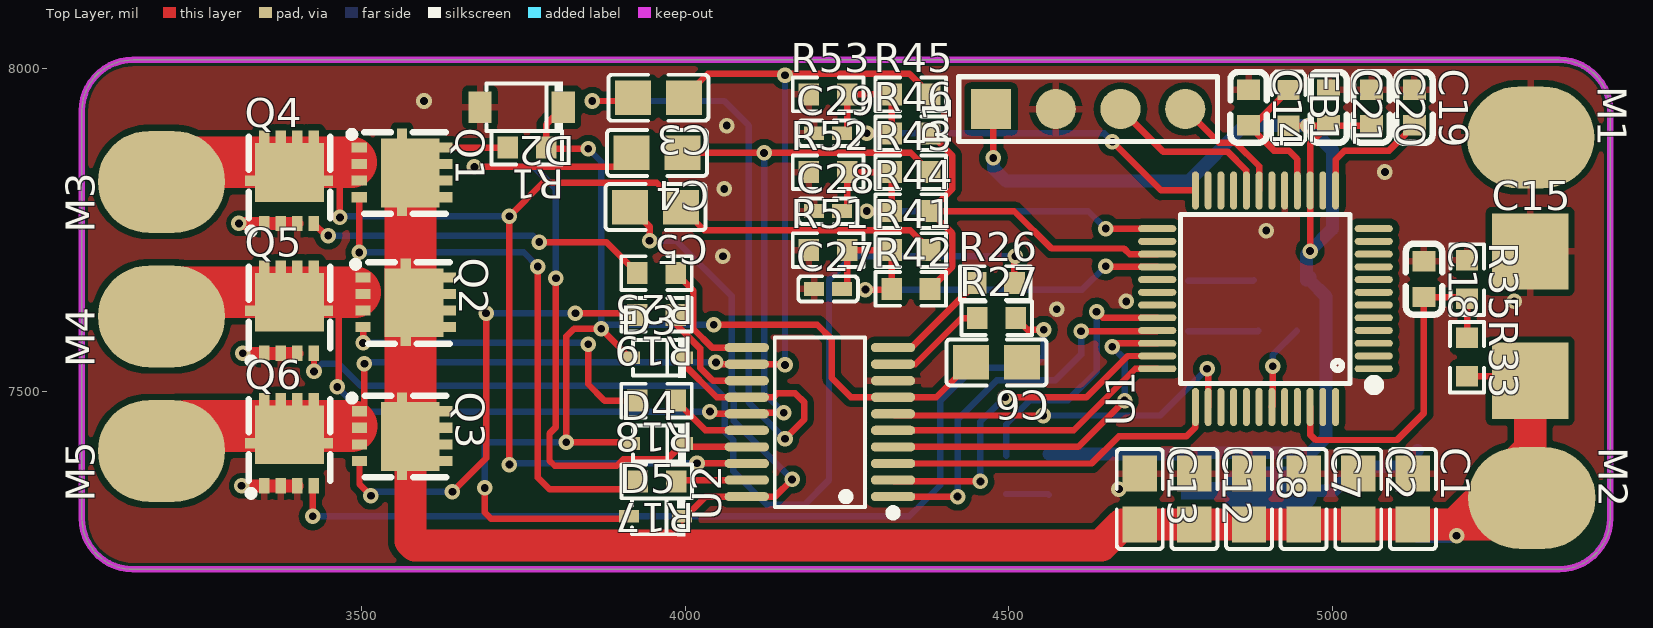
[diagram p0: Top Layer view]
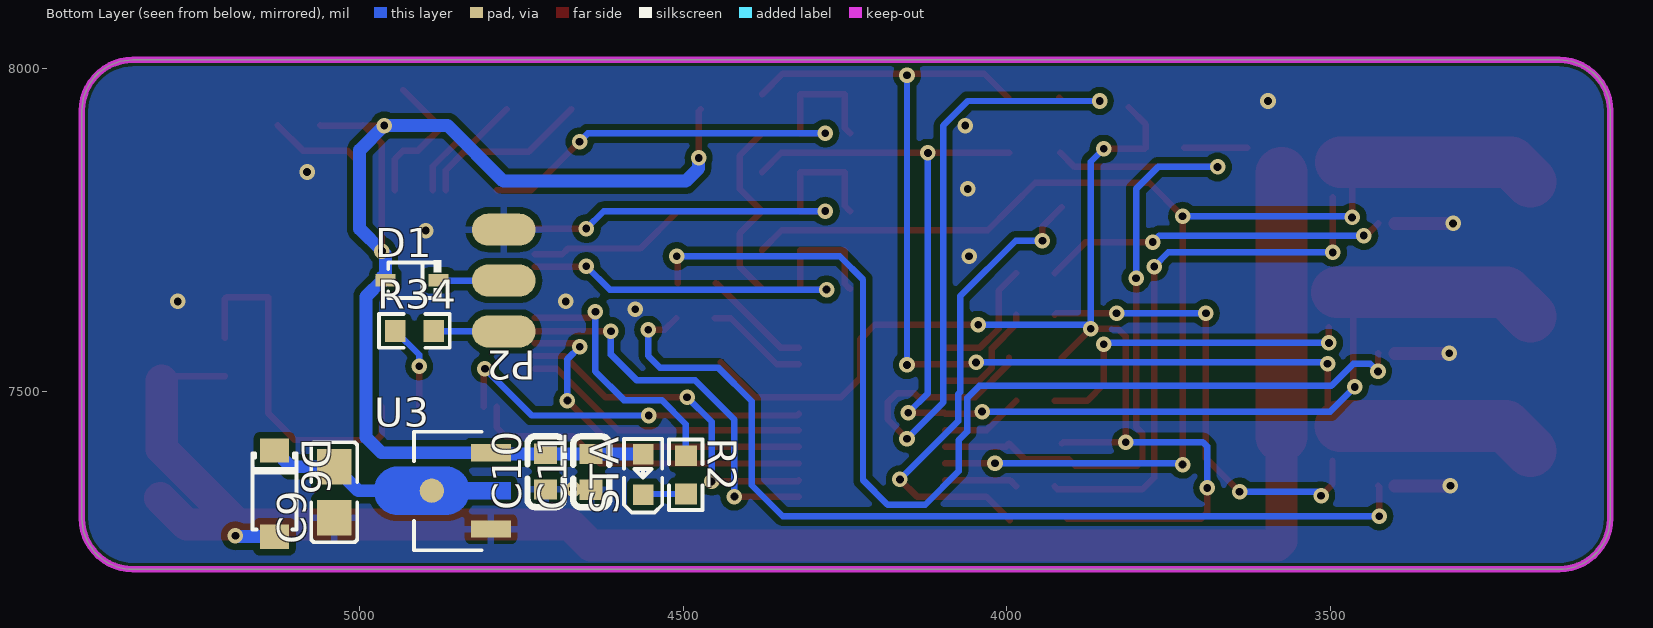
[diagram p1: Bottom Layer view, seen from below]
# Altium PCB MISC52085.pcbdoc
Units mil, origin at the board's own origin, x right, y up, seen from the top; angles counter-clockwise.
Board outline 2362.2 x 787.4 mil, 2 copper layers (Top Layer, Bottom Layer), stack 62.206 mil thick; 66 components, 45 nets, 249 pads, 70 vias.

## Layer stack, top to bottom
Top Solder Mask Layer: solder mask 0.394, Dk 3.3
Top Layer: signal copper 1.379
Dielectric1: surface 59.449, FR4, Dk 4.5
Bottom Layer: signal copper 1.378
Bottom Solder Mask Layer: solder mask 0.394, Dk 3.3

## Board outline
3067.18,7304.15 ccw(c3145.92,7304.15) 3145.92,7225.41 5350.64,7225.41 ccw(c5350.64,7304.15) 5429.38,7304.15 5429.38,7934.07 ccw(c5350.64,7934.07) 5350.64,8012.81 3145.92,8012.81 ccw(c3145.92,7934.07) 3067.18,7934.07

## Design rules (kind name [scope] priority, off if disabled: settings)
BoardOutlineClearance copperThickness2oz_1 [All] p2 off: genericclearance=7.99 ignorepadtopadclearanceinfootprint=FALSE except(0: Arc-SplitContinuation Track-SplitContinuation SMDPad-SplitContinuation THPad-SplitContinuation Via-SplitContinuation Fill-SplitContinuation Region-SplitContinuation Poly-SplitContinuation Text-SplitContinuation Hole-SplitContinuation; 5.98: Arc-CutoutEdge Track-CutoutEdge SMDPad-CutoutEdge THPad-CutoutEdge Via-CutoutEdge Text-CutoutEdge; 6.89: Hole-OutlineEdge Hole-CutoutEdge; 10: Poly-OutlineEdge Poly-CutoutEdge; 11.81: Arc-OutlineEdge Track-OutlineEdge SMDPad-OutlineEdge THPad-OutlineEdge Via-OutlineEdge Fill-OutlineEdge Region-OutlineEdge Text-OutlineEdge Fill-CutoutEdge Region-CutoutEdge)
BoardOutlineClearance Plane_innerPlane_1 [All] p4 off: genericclearance=4.02 ignorepadtopadclearanceinfootprint=FALSE except(0: Arc-SplitContinuation Track-SplitContinuation SMDPad-SplitContinuation THPad-SplitContinuation Via-SplitContinuation Fill-SplitContinuation Region-SplitContinuation Poly-SplitContinuation Text-SplitContinuation Hole-SplitContinuation; 5.98: Arc-CutoutEdge Track-CutoutEdge SMDPad-CutoutEdge THPad-CutoutEdge Via-CutoutEdge Text-CutoutEdge; 6.89: Hole-OutlineEdge Hole-CutoutEdge; 10: Poly-OutlineEdge Poly-CutoutEdge; 11.81: Arc-OutlineEdge Track-OutlineEdge SMDPad-OutlineEdge THPad-OutlineEdge Via-OutlineEdge Fill-OutlineEdge Region-OutlineEdge Text-OutlineEdge Fill-CutoutEdge Region-CutoutEdge)
BoardOutlineClearance Copper_copperRegion_1 [All] p6 off: genericclearance=4.02 ignorepadtopadclearanceinfootprint=FALSE except(0: Arc-SplitContinuation Track-SplitContinuation SMDPad-SplitContinuation THPad-SplitContinuation Via-SplitContinuation Fill-SplitContinuation Region-SplitContinuation Poly-SplitContinuation Text-SplitContinuation Hole-SplitContinuation; 5.98: Arc-CutoutEdge Track-CutoutEdge SMDPad-CutoutEdge THPad-CutoutEdge Via-CutoutEdge Text-CutoutEdge; 6.89: Hole-OutlineEdge Hole-CutoutEdge; 10: Poly-OutlineEdge Poly-CutoutEdge; 11.81: Arc-OutlineEdge Track-OutlineEdge SMDPad-OutlineEdge THPad-OutlineEdge Via-OutlineEdge Fill-OutlineEdge Region-OutlineEdge Text-OutlineEdge Fill-CutoutEdge Region-CutoutEdge)
BoardOutlineClearance copperThickness1oz_1 [All] p8: genericclearance=4.02 ignorepadtopadclearanceinfootprint=FALSE except(0: Arc-SplitContinuation Track-SplitContinuation SMDPad-SplitContinuation THPad-SplitContinuation Via-SplitContinuation Fill-SplitContinuation Region-SplitContinuation Poly-SplitContinuation Text-SplitContinuation Hole-SplitContinuation; 5.98: Arc-CutoutEdge Track-CutoutEdge SMDPad-CutoutEdge THPad-CutoutEdge Via-CutoutEdge Text-CutoutEdge; 6.89: Hole-OutlineEdge Hole-CutoutEdge; 10: Poly-OutlineEdge Poly-CutoutEdge; 11.81: Arc-OutlineEdge Track-OutlineEdge SMDPad-OutlineEdge THPad-OutlineEdge Via-OutlineEdge Fill-OutlineEdge Region-OutlineEdge Text-OutlineEdge Fill-CutoutEdge Region-CutoutEdge)
Clearance copperThickness2oz [All] p1 off: gap=7.99 ignorepadtopadclearanceinfootprint=FALSE except(5.98: SMDPad-Track SMDPad-SMDPad THPad-Track SMDPad-THPad THPad-THPad Track-Via SMDPad-Via THPad-Via Via-Via Fill-SMDPad Region-SMDPad Fill-THPad Region-THPad Fill-Via Region-Via Fill-Fill Fill-Region Region-Region Arc-Track Arc-SMDPad Arc-THPad Arc-Via Fill-Arc Region-Arc Arc-Arc Text-Track SMDPad-Text Text-THPad Text-Via Fill-Text Region-Text Arc-Text Text-Text; 6.89: Hole-Track Hole-SMDPad Hole-THPad Hole-Via Fill-Hole Region-Hole Hole-Arc Hole-Text; 10: Poly-Track Poly-SMDPad Poly-THPad Poly-Via Poly-Fill Poly-Region Poly-Poly Poly-Arc Poly-Text Poly-Hole; 11.81: Fill-Track Region-Track)
Clearance Plane_innerPlane [All] p3 off: gap=4.02 ignorepadtopadclearanceinfootprint=FALSE except(5.98: SMDPad-Track SMDPad-SMDPad THPad-Track SMDPad-THPad THPad-THPad Track-Via SMDPad-Via THPad-Via Via-Via Fill-SMDPad Region-SMDPad Fill-THPad Region-THPad Fill-Via Region-Via Fill-Fill Fill-Region Region-Region Arc-Track Arc-SMDPad Arc-THPad Arc-Via Fill-Arc Region-Arc Arc-Arc Text-Track SMDPad-Text Text-THPad Text-Via Fill-Text Region-Text Arc-Text Text-Text; 6.89: Hole-Track Hole-SMDPad Hole-THPad Hole-Via Fill-Hole Region-Hole Hole-Arc Hole-Text; 10: Poly-Track Poly-SMDPad Poly-THPad Poly-Via Poly-Fill Poly-Region Poly-Poly Poly-Arc Poly-Text Poly-Hole; 11.81: Fill-Track Region-Track)
Clearance Copper_copperRegion [All] p5 off: gap=4.02 ignorepadtopadclearanceinfootprint=FALSE except(5.98: SMDPad-Track SMDPad-SMDPad THPad-Track SMDPad-THPad THPad-THPad Track-Via SMDPad-Via THPad-Via Via-Via Fill-SMDPad Region-SMDPad Fill-THPad Region-THPad Fill-Via Region-Via Fill-Fill Fill-Region Region-Region Arc-Track Arc-SMDPad Arc-THPad Arc-Via Fill-Arc Region-Arc Arc-Arc Text-Track SMDPad-Text Text-THPad Text-Via Fill-Text Region-Text Arc-Text Text-Text; 6.89: Hole-Track Hole-SMDPad Hole-THPad Hole-Via Fill-Hole Region-Hole Hole-Arc Hole-Text; 10: Poly-Track Poly-SMDPad Poly-THPad Poly-Via Poly-Fill Poly-Region Poly-Poly Poly-Arc Poly-Text Poly-Hole; 11.81: Fill-Track Region-Track)
Clearance copperThickness1oz [All] p7: gap=4.02 ignorepadtopadclearanceinfootprint=FALSE except(5.98: SMDPad-Track SMDPad-SMDPad THPad-Track SMDPad-THPad THPad-THPad Track-Via SMDPad-Via THPad-Via Via-Via Fill-SMDPad Region-SMDPad Fill-THPad Region-THPad Fill-Via Region-Via Fill-Fill Fill-Region Region-Region Arc-Track Arc-SMDPad Arc-THPad Arc-Via Fill-Arc Region-Arc Arc-Arc Text-Track SMDPad-Text Text-THPad Text-Via Fill-Text Region-Text Arc-Text Text-Text; 6.89: Hole-Track Hole-SMDPad Hole-THPad Hole-Via Fill-Hole Region-Hole Hole-Arc Hole-Text; 10: Poly-Track Poly-SMDPad Poly-THPad Poly-Via Poly-Fill Poly-Region Poly-Poly Poly-Arc Poly-Text Poly-Hole; 11.81: Fill-Track Region-Track)
DiffPairsRouting differentialPair [All] p1: maxlimit=6 minlimit=6 mostfreqgap=6 toplayer_minwidth=5 toplayer_prefwidth=10 toplayer_maxwidth=100 toplayer_mingap=6 toplayer_prefgap=6 toplayer_maxgap=6 bottomlayer_minwidth=5 bottomlayer_prefwidth=10 bottomlayer_maxwidth=100 bottomlayer_mingap=6 bottomlayer_prefgap=6 bottomlayer_maxgap=6 maxuncoupledlength=10
HoleToHoleClearance otherClearance [All] p1: gap=11.81 allowstackedmicrovias=TRUE
Length netLength [All] p1: minlimit=0 maxlimit=0
PasteMaskExpansion pasteMaskExpansion [All] p1: expansion=0
PlaneConnect innerPlane [All] p1: planeconnectstyle=Relief reliefexpansion=20 reliefentries=4 reliefconductorwidth=10 reliefairgap=10
PolygonConnect copperRegion [All] p1: connectstyle=Relief reliefconductorwidth=10 reliefentries=4 polygonreliefangle="90 Angle" airgapwidth=10 via.connectstyle=Relief via.reliefconductorwidth=10 via.reliefentries=4 via.polygonreliefangle="90 Angle" via.airgapwidth=10
RoutingVias viaSize [All] p1: holewidth=12.01 width=24.02 viastyle="Through Hole" minholewidth=11.81 minwidth=19.68 maxholewidth=248.03 maxwidth=393.7
SolderMaskExpansion solderMaskExpansion [IsVia] p1: expansion=-1000 istentingtop=TRUE
SolderMaskExpansion solderMaskExpansion [All] p2: expansion=2.01 istentingtop=FALSE
Width copperThickness2oz_2 [All] p1 off: maxlimit=100 minlimit=8 preferedwidth=10
Width copperThickness1oz_2 [All] p2: maxlimit=100 minlimit=5 preferedwidth=10

## Components (designator, comment, footprint, x,y, rotation, side; value= is the part's Value field where it differs from the comment)
C1 "22uF" C0805 5124.51,7333.92 r270 top
C2 "22uF" C0805 5040.09,7333.92 r270 top
C3 "4.7uF" C0805 3958.24,7954.26 r180 top
C4 "4.7uF" C0805 3956.24,7869.04 r180 top
C5 "4.7uF" C0805 3954,7785.25 r180 top
C6 "22uF" C0805 4481.05,7545.28 r180 top
C7 "22uF" C0805 4955.66,7333.92 r270 top
C8 "22uF" C0805 4871.23,7333.92 r270 top
C9 "22uF" C0805 5039.24,7344.49 r90 bottom
C10 "10uF" C0603 4712.62,7376.35 r90 bottom
C11 "100nF" C0603 4642.14,7376.1 r90 bottom
C12 "22uF" C0805 4786.8,7333.92 r270 top
C13 "22uF" C0805 4702.37,7333.92 r270 top
C14 "100nF" C0603 4870.51,7939.35 r270 top
C15 "470uf" 焊盘 5305.72,7516.65 r0 top
C18 "100nF" C0603 5141.64,7673.78 r270 top
C19 "100nF" C0603 5126.94,7939.35 r270 top
C20 "10uF" C0603 5060.66,7939.35 r270 top
C21 "100nF" C0603 4994.38,7939.35 r270 top
C27 "100nF" C0402 4220.55,7658.77 r0 top
C28 "100nF" C0402 4220.55,7779.02 r0 top
C29 "100nF" C0402 4220.55,7899.28 r0 top
D1 "B5819WS" SOD-323_L1.7-W1.3-LS2.5-FD 4919.31,7672.15 r180 bottom
D2 "BZT52C15" SOD-123_L2.7-W1.6-LS3.7-RD 3747,7939.55 r180 top
D3 "B5819WS" SOD-323_L1.7-W1.3-LS2.5-FD 3955.39,7552.38 r0 top
D4 "B5819WS" SOD-323_L1.7-W1.3-LS2.5-FD 3955.39,7419.82 r0 top
D5 "B5819WS" SOD-323_L1.7-W1.3-LS2.5-FD 3954,7307.25 r0 top
D6 "DSK34" SOD-123_L2.8-W1.8-LS3.7-RD 5131.61,7342.48 r270 bottom
FB1 "MLB1608F-000T" L0603 4932.48,7938.69 r270 top
M1 "MountHole" 3*4焊盘 5306.45,7892.98 r270 top
M2 "MountHole" 3*4焊盘 5308.45,7335.61 r270 top
M3 "MountHole" 3*4焊盘 3190.27,7824.24 r90 top
M4 "MountHole" 3*4焊盘 3190.27,7616.24 r90 top
M5 "MountHole" 3*4焊盘 3190.27,7408.25 r90 top
P1 "Header-D-M 1x4P" 调试端口2.54_1X4 4617.58,7936.82 r90 top
P2 "Header-D-M 1x3P" 3P 4777.16,7671.73 r0 bottom
Q1 "TPN2R703NL,L1Q(M" TSON-8_L3.1-W3.1-P0.65-LS3.3-BL-EP 3561.99,7838.93 r270 top
Q2 "TPN2R703NL,L1Q(M" TSON-8_L3.1-W3.1-P0.65-LS3.3-BL-EP 3567.75,7638.14 r270 top
Q3 "TPN2R703NL,L1Q(M" TSON-8_L3.1-W3.1-P0.65-LS3.3-BL-EP 3562.24,7431.33 r270 top
Q4 "TPN2R703NL,L1Q(M" TSON-8_L3.1-W3.1-P0.65-LS3.3-BL-EP 3387.35,7825.95 r0 top
Q5 "TPN2R703NL,L1Q(M" TSON-8_L3.1-W3.1-P0.65-LS3.3-BL-EP 3387.35,7625.16 r0 top
Q6 "TPN2R703NL,L1Q(M" TSON-8_L3.1-W3.1-P0.65-LS3.3-BL-EP 3387.35,7420.36 r0 top
R1 "100Ω" R0603 3755.03,7877.3 r180 top
R2 "10kΩ" R0603 4495.84,7371.45 r270 bottom
R17 "4.7Ω" R0603 3956,7361.25 r180 top
R18 "4.7Ω" R0603 3955.39,7486.1 r180 top
R19 "4.7Ω" R0603 3955.39,7618.67 r180 top
R25 "4.7Ω" R0603 3955.39,7683.25 r180 top
R26 "4.7Ω" R0603 4479.04,7667.76 r0 top
R27 "4.7Ω" R0603 4481.05,7613.55 r0 top
R33 "47kΩ" R0603 5208.15,7553.3 r270 top
R34 "100Ω" R0603 4915.29,7593.84 r180 bottom
R35 "10kΩ" R0603 5208.36,7673.26 r270 top
R41 "5.1kΩ" R0603 4348.46,7718.9 r0 top
R42 "1kΩ" R0603 4348.46,7658.77 r0 top
R43 "5.1kΩ" R0603 4348.46,7839.15 r0 top
R44 "1kΩ" R0603 4348.46,7779.02 r0 top
R45 "5.1kΩ" R0603 4348.46,7959.41 r0 top
R46 "1kΩ" R0603 4348.46,7899.28 r0 top
R51 "1kΩ" R0603 4220.55,7718.9 r0 top
R52 "1kΩ" R0603 4220.55,7839.15 r0 top
R53 "1kΩ" R0603 4220.55,7959.41 r0 top
STA "LTST-C191KSKT" LED0603-RD-YELLOW 4561.65,7371.97 r90 bottom
U1 "STC32G8K64-42I-LQFP48" LQFP-48_L7.0-W7.0-P0.50-LS9.0-BL 4896.68,7643.66 r90 top
U2 "FD6288T" TSSOP-20_L6.5-W4.4-P0.65-LS6.4-BL 4207.97,7452.91 r90 top
U3 "SE8650KX-LF" SOT-89-3_L4.3-W2.3-P1.50-LS4.3-BR 4850.5,7346.5 r180 bottom

## Footprints (in the part's own frame and the unit in brackets; to place one, negate y for a bottom-side part, rotate by r counter-clockwise, add the part's x,y. Pads: shape width x height; smd on the part's side, far side on the other; paste and mask are expansions set on the pad)
3*4焊盘 [mm]
  oval 4x5 smd paste+0 mask+0.102: 1(0,0)
3P [mm]
  oval 2.5x1.25 smd paste+0 mask+0.051: 1(0,2) 2(0,0) 3(0,-2)
C0402 [mm]
  rect 0.79x0.54 smd paste-100 mask+0.051: 1(-0.545,0) 2(0.545,0)
  silkscreen extent -1.17,-0.5 1.17,0.5
C0603 [mm]
  rect 0.8x0.9 smd: 1(-0.7,0) 2(0.7,0)
  silkscreen extent -1.39,-0.71 1.39,0.71
C0805 [mm]
  rect 1.41x1.35 smd paste-100 mask+0.051: 1(-1,0) 2(1,0)
  silkscreen extent -1.96,-0.9 1.96,0.9
L0603 [mm]
  rect 0.8x0.864 smd paste-100 mask+0.051: 1(-0.7,0) 2(0.7,0)
  silkscreen extent -1.42,-0.65 1.42,0.65
LED0603-RD-YELLOW [mm]
  rect 0.8x0.8 smd: 1(-0.799,-0.003) 2(0.799,0.003)
  silkscreen extent -1.49,-0.75 1.39,0.76
LQFP-48_L7.0-W7.0-P0.50-LS9.0-BL [mm]
  oval 0.27x1.5 smd paste+0 mask+0.05: 1(-2.75,-4.25) 2(-2.25,-4.25) 3(-1.75,-4.25) 4(-1.25,-4.25) 5(-0.75,-4.25) 6(-0.25,-4.25) 7(0.25,-4.25) 8(0.75,-4.25) 9(1.25,-4.25) 10(1.75,-4.25) 11(2.25,-4.25) 12(2.75,-4.25) 25(2.75,4.25) 26(2.25,4.25) 27(1.75,4.25) 28(1.25,4.25) 29(0.75,4.25) 30(0.25,4.25) 31(-0.25,4.25) 32(-0.75,4.25) 33(-1.25,4.25) 34(-1.75,4.25) 35(-2.25,4.25) 36(-2.75,4.25)
  oval 1.5x0.27 smd paste+0 mask+0.05: 13(4.25,-2.75) 14(4.25,-2.25) 15(4.25,-1.75) 16(4.25,-1.25) 17(4.25,-0.75) 18(4.25,-0.25) 19(4.25,0.25) 20(4.25,0.75) 21(4.25,1.25) 22(4.25,1.75) 23(4.25,2.25) 24(4.25,2.75) 37(-4.25,2.75) 38(-4.25,2.25) 39(-4.25,1.75) 40(-4.25,1.25) 41(-4.25,0.75) 42(-4.25,0.25) 43(-4.25,-0.25) 44(-4.25,-0.75) 45(-4.25,-1.25) 46(-4.25,-1.75) 47(-4.25,-2.25) 48(-4.25,-2.75)
  silkscreen extent -3.59,-4.46 3.3,3.34
R0603 [mil]
  rect 31.75x34.02 smd paste-3937.01 mask+2: 1(-29.66,0) 2(29.66,0)
  silkscreen extent -55,-26 55,26
SOD-123_L2.7-W1.6-LS3.7-RD [mm]
  rect 0.91x1.22 smd: 1(-1.635,0) 2(1.635,0)
  silkscreen extent -1.6,-1 1.38,1
SOD-123_L2.8-W1.8-LS3.7-RD [mm]
  rect 0.95x1.15 smd: 1(-1.692,0) 2(1.692,0)
  silkscreen extent -1.58,-0.87 1.41,0.87
SOD-323_L1.7-W1.3-LS2.5-FD [mm]
  rect 0.78x0.5 smd: 1(-1.04,0) 2(1.04,0)
  silkscreen extent -0.93,-0.78 1.15,0.78
SOT-89-3_L4.3-W2.3-P1.50-LS4.3-BR [mm]
  rect 1.575x0.672 smd: 1(1.356,-1.5) 3(1.356,1.5)
  round 0.95 smd: 2(-0.966,0.009)
  Top Layer region: -2.283,0.959 -0.429,0.959 -0.384,0.958 -0.34,0.955 -0.296,0.949 -0.252,0.942 -0.208,0.933 -0.165,0.921 -0.123,0.908 -0.081,0.893 -0.04,0.875 0,0.856 0.04,0.835 0.078,0.812 0.115,0.788 0.151,0.761 0.185,0.733 0.219,0.704 0.251,0.673 0.281,0.64 0.31,0.606 0.337,0.571 0.362,0.534 0.386,0.497 0.408,0.458 0.428,0.418 0.447,0.339 2.144,0.339 2.144,-0.321 0.447,-0.321 0.428,-0.401 0.408,-0.44 0.386,-0.479 0.362,-0.517 0.337,-0.553 0.31,-0.588 0.281,-0.622 0.251,-0.655 0.219,-0.686 0.185,-0.716 0.151,-0.744 0.115,-0.77 0.078,-0.795 0.04,-0.818 0,-0.839 -0.04,-0.858 -0.081,-0.875 -0.123,-0.89 -0.165,-0.904 -0.208,-0.915 -0.252,-0.925 -0.296,-0.932 -0.34,-0.937 -0.384,-0.94 -0.429,-0.941 -2.283,-0.941 -2.328,-0.94 -2.372,-0.937 -2.416,-0.932 -2.46,-0.925 -2.504,-0.915 -2.547,-0.904 -2.589,-0.89 -2.631,-0.875 -2.672,-0.858 -2.713,-0.839 -2.752,-0.818 -2.79,-0.795 -2.827,-0.77 -2.863,-0.744 -2.898,-0.716 -2.931,-0.686 -2.963,-0.655 -2.993,-0.622 -3.022,-0.588 -3.049,-0.553 -3.075,-0.517 -3.098,-0.479 -3.12,-0.44 -3.141,-0.401 -3.159,-0.36 -3.175,-0.318 -3.189,-0.276 -3.202,-0.233 -3.212,-0.19 -3.22,-0.146 -3.227,-0.102 -3.231,-0.058 -3.233,-0.013 -3.233,0.031 -3.231,0.076 -3.227,0.12 -3.22,0.164 -3.212,0.208 -3.202,0.251 -3.189,0.294 -3.175,0.336 -3.159,0.377 -3.141,0.418 -3.12,0.458 -3.098,0.497 -3.075,0.534 -3.049,0.571 -3.022,0.606 -2.993,0.64 -2.963,0.673 -2.931,0.704 -2.898,0.733 -2.863,0.761 -2.827,0.788 -2.79,0.812 -2.752,0.835 -2.713,0.856 -2.672,0.875 -2.631,0.893 -2.589,0.908 -2.547,0.921 -2.504,0.933 -2.46,0.942 -2.416,0.949 -2.372,0.955 -2.328,0.958
  silkscreen extent -1.66,-2.33 0.99,2.33
TSON-8_L3.1-W3.1-P0.65-LS3.3-BL-EP [mm]
  rect 0.4x0.6 smd paste-100 mask+0.051: 1(-0.975,-1.675) 2(-0.325,-1.675) 3(0.325,-1.675) 4(0.975,-1.675) 5(0.975,1.675) 6(0.325,1.675) 7(-0.325,1.675) 8(-0.975,1.675)
  rect 0.6x0.4 smd paste-100 mask+0.051: 9(-1.42,0) 9(1.42,0)
  rect 2.7x2.3 smd paste-100 mask+0.051: 9(0.02,0.325)
  silkscreen extent -1.62,-2.1 1.62,1.72
TSSOP-20_L6.5-W4.4-P0.65-LS6.4-BL [mil]
  oval 14.33x68.58 smd: 1(-115.16,-113.03) 2(-89.57,-113.03) 3(-63.98,-113.03) 4(-38.39,-113.03) 5(-12.79,-113.03) 6(12.8,-113.03) 7(38.39,-113.03) 8(63.98,-113.03) 9(89.57,-113.03) 10(115.16,-113.03) 11(115.16,113.03) 12(89.57,113.03) 13(63.98,113.03) 14(38.39,113.03) 15(12.8,113.03) 16(-12.79,113.03) 17(-38.39,113.03) 18(-63.98,113.03) 19(-89.57,113.03) 20(-115.16,113.03)
  silkscreen extent -146,-119 131,70
焊盘 [mm]
  rect 3x3 smd paste+0 mask+0.051: 1(0,0) 2(0,5.08)
调试端口2.54_1X4 [mil]
  rect 62x62 smd paste+0 mask+2: 1(0,145)
  round 62 smd paste+0 mask+2: 2(0,45) 3(0,-55) 4(0,-155)
  silkscreen extent -50,-205 50,195

## Via types
v1: diameter 24.02, hole 12, Top Layer to Bottom Layer, 70 vias

## Nets (pads, with @x,y where several pads share a name; then routed paths per layer and width w, separated by ;. In a path a pad name is that pad's centre, name@x,y a point inside that pad or via, vN(x,y) a via of type N, cw(c..) or ccw(c..) an arc to the next point about the centre after c; other vN are vias at no path point)
$1N789: C14.2 FB1.1 U1.16 | length 230.1
  Top Layer w10: FB1.1 4878.02,7911.79 C14.2 4909.73,7872.57 4932.82,7872.57 4945.89,7859.5 U1.16
$1N2255: C6.2 D2.1 D3.1 D4.1 D5.1 R1.1 U2.7 | length 1940.1
  Top Layer w10: v1(3690,7351.25) 3690,7313.25 3700,7303.25 D5.1@3906.45,7303.25 ; D2.1 3784.69,7912.86 R1.1 3786.74,7875.25 v1(3850,7875.25) ; D4.1 3912.45,7421.82 v1(3816,7421.82) 3816,7585.25 3828,7597.25 v1(3870,7597.25) 3870,7596.84 D3.1 ; v1(4044,7603.25) 4204,7603.25 4226,7581.25 4226,7521.25 4255.95,7491.3 U2.7 4387.7,7491.3 C6.2
  Bottom Layer w10: v1(3690,7351.25) 3690,7415.25 3696.57,7421.82 v1(3816,7421.82) ; v1(3850,7875.25) 3870,7855.25 v1(3870,7597.25) 3876,7603.25 v1(4044,7603.25)
$1N2771: R2.2 STA.1 | length 66.2
  Bottom Layer w10: R2.2 4560.21,7341.79 STA.1
$1N2815: D1.2 P2.2 | length 101.4
  Bottom Layer w10: P2.2 4877.95,7671.73 D1.2
$1N2868: P2.1 R34.2 | length 108.8
  Bottom Layer w10: P2.1 4884.78,7592.99 R34.2
$1N3796: C9.2 D6.1 U3.2 | length 253.5
  Bottom Layer w20: U3.2@4903.89,7346.84 5002.22,7346.84 C9.2 5106.35,7383.86 D6.1
$1N4847: Q1.4 R17.2 | length 859.3
  Top Layer w10: v1(3496.05,7715.25) Q1.4 ; v1(3772,7693.25) 3772,7367.25 3790,7349.25 3921.45,7349.25 R17.2@3925.73,7353.53
  Bottom Layer w10: v1(3496.05,7715.25) 3750,7715.25 v1(3772,7693.25)
$1N4886: Q4.4 R25.2 | length 531.8
  Top Layer w10: Q4.4 3444.49,7741.25 v1(3448,7741.25) ; v1(3774,7731.25) 3877.73,7731.25 R25.2
  Bottom Layer w10: v1(3448,7741.25) 3764,7741.25 v1(3774,7731.25)
$1N6016: Q2.4 R18.2 | length 521.7
  Top Layer w10: v1(3501.81,7575.25) Q2.4 ; v1(3850,7573.25) 3850,7511.25 3875.15,7486.1 R18.2
  Bottom Layer w10: v1(3501.81,7575.25) 3848,7575.25 v1(3850,7573.25)
$1N6018: Q5.4 R26.2 | length 1648.6
  Top Layer w10: Q5.4 3426,7558.95 v1(3426,7531.25) ; R26.2 4508.7,7707.95 v1(4510,7709.25)
  Bottom Layer w10: v1(3426,7531.25) 3438,7543.25 3464,7543.25 3498,7509.25 4042,7509.25 4060.99,7490.26 4060.99,7438.26 4074,7425.25 4074,7377.25 4126,7325.25 4184,7325.25 4222,7363.25 4222,7673.25 4258,7709.25 v1(4510,7709.25)
$1N6264: Q3.4 R19.2 | length 721.9
  Top Layer w10: Q3.4 3496.29,7356.96 v1(3514,7339.25) ; v1(3640,7345.25) 3692,7397.25 v1(3692,7621.25) ; v1(3830,7621.25) 3923.15,7621.25 R19.2
  Bottom Layer w10: v1(3514,7339.25) 3520,7345.25 v1(3640,7345.25) ; v1(3692,7621.25) v1(3830,7621.25)
$1N6266: Q6.4 R27.2 | length 1447.8
  Top Layer w10: v1(3424,7307.25) 3424,7352.68 Q6.4 ; R27.2 4528.71,7595.55 v1(4554,7595.55)
  Bottom Layer w10: v1(3424,7307.25) 4346,7307.25 4394,7355.25 4394,7485.25 4446,7537.25 4536,7537.25 4554,7555.25 v1(4554,7595.55)
ABMF: C27.2 R41.1 R42.1 R51.2 U1.28 | length 699.7
  Top Layer w10: C27.2 4250.21,7666.97 R51.2 R41.1 R42.1 4317.75,7657.72 v1(4278.25,7657.72) ; v1(4649.71,7693.86) 4650.7,7692.87 U1.28
  Bottom Layer w10: v1(4278.25,7657.72) 4613.57,7657.72 v1(4649.71,7693.86)
BATADC: C18.2 R33.1 R35.2 U1.46 | length 547.3
  Top Layer w10: U1.46 4965.58,7433.67 4974,7425.25 5100,7425.25 5141.64,7466.9 C18.2 5205.74,7646.22 R35.2 5208.36,7583.17 R33.1
BBMF: C28.2 R43.1 R44.1 R52.2 U1.25 | length 691.1
  Top Layer w10: C28.2 4250.21,7787.22 R52.2 R43.1 R44.1 v1(4280.26,7779.02) ; v1(4649.71,7752.09) 4729.2,7752.09 U1.25
  Bottom Layer w10: v1(4280.26,7779.02) 4622.78,7779.02 v1(4649.71,7752.09)
CBMF: C29.2 R45.1 R46.1 R53.2 U1.24 | length 775.5
  Top Layer w10: C29.2 4250.21,7907.48 R53.2 R45.1 R46.1 v1(4280.26,7899.28) ; v1(4660.08,7886.33) 4735.42,7810.98 U1.24
  Bottom Layer w10: v1(4280.26,7899.28) 4647.13,7899.28 v1(4660.08,7886.33)
CMPO: U1.23
DBRX: P1.4 U1.19 | length 188.2
  Top Layer w10: P1.4 4824.35,7885.05 4850.06,7885.05 4886.84,7848.27 U1.19
DBTX: P1.3 U1.20 | length 264.8
  Top Layer w10: P1.3 4738.36,7871.04 4837.97,7871.04 4867.15,7841.86 U1.20
GND: C1.1 C2.1 C6.1 C7.1 C8.1 C9.1 C10.1 C11.1 C12.1 C13.1 C14.1 C15.2 C18.1 C19.1 C20.1 C21.1 C27.1 C28.1 C29.1 D2.2 M1.1 P1.2 P2.3 Q4.1 Q4.2 Q4.3 Q5.1 Q5.2 Q5.3 Q6.1 Q6.2 Q6.3 R35.1 R51.1 R52.1 R53.1 U1.17 U2.8 U3.1 | length 260.4
  Top Layer w20: v1(3310,7760.01) Q4.1 Q4.2 Q4.3 ; v1(3314,7354.41) Q6.1 Q6.2 Q6.3 ; v1(3316,7559.22) Q5.1 Q5.2 Q5.3
  other v1: 4670.09,7349.32 4574,7627.25 4681.28,7639.51 5281.28,7639.51 4058,7709.25 4897.67,7748.98 4060,7813.25 5081.28,7839.51 4064,7911.25 3596,7949.25
HOA: R17.1 U2.19 | length 113.9
  Top Layer w10: R17.1@3985.05,7353.53 3994.86,7363.34 U2.19
HOB: R18.1 U2.16 | length 128.9
  Top Layer w10: R18.1 4031.03,7440.12 U2.16
HOC: R19.1 U2.13 | length 177.9
  Top Layer w10: R19.1 3985.05,7604.39 4022.67,7566.78 4022.67,7536.91 4042.69,7516.89 U2.13
LED: R2.1 U1.32 | length 412.1
  Top Layer w10: v1(4635.65,7623.59) 4645.1,7614.13 U1.32
  Bottom Layer w10: R2.1 4495.84,7449.64 4533.25,7487.05 4591.48,7487.05 4635.65,7531.22 v1(4635.65,7623.59)
LOA: R25.1 U2.11 | length 192.2
  Top Layer w10: R25.1 4012,7656.31 4012,7597.27 4041.2,7568.07 U2.11
LOB: R26.1 U2.10 | length 169.7
  Top Layer w10: U2.10 4349.69,7568.07 R26.1
LOC: R27.1 U2.9 | length 159.8
  Top Layer w10: U2.9 4355.23,7542.48 4426.3,7613.55 R27.1
MID: R42.2 R44.2 R46.2 U1.27 | length 676.7
  Top Layer w10: R42.2 4412.78,7693.43 4412.78,7744.36 R44.2 ; R46.2 4412.78,7864.62 4412.78,7813.69 R44.2 ; U1.27 4686.69,7712.56 4678,7721.25 4566,7721.25 4508.23,7779.02 R44.2
P1.0: U1.5
PWMAH: U1.33 U2.1 | length 605.7
  Top Layer w10: U2.1 v1(4420.81,7337.75) ; v1(4611.56,7593.47) 4728.37,7593.47 U1.33
  Bottom Layer w10: v1(4420.81,7337.75) 4420.81,7456.93 4481.13,7517.25 4571.49,7517.25 4611.56,7557.32 v1(4611.56,7593.47)
PWMAL: U1.34 U2.4 | length 550.4
  Top Layer w10: U2.4 4607.22,7414.52 v1(4678.81,7486.11) ; v1(4659.8,7569.36) 4665.21,7574.76 U1.34
  Bottom Layer w10: v1(4659.8,7569.36) 4678.81,7550.35 v1(4678.81,7486.11)
PWMBH: U1.35 U2.2 | length 543.4
  Top Layer w10: U2.2 4323.09,7361.25 v1(4456,7361.25) ; v1(4494,7491.25) 4620,7491.25 4683.83,7555.08 U1.35
  Bottom Layer w10: v1(4456,7361.25) 4456,7453.25 v1(4494,7491.25)
PWMBL: U1.36 U2.5 | length 447.8
  Top Layer w10: U2.5 4600.31,7440.12 4695.58,7535.39 U1.36
PWMCH: U1.37 U2.3 | length 522
  Top Layer w10: U2.3 4627.9,7388.93 4669.79,7430.83 4774.2,7430.83 4788.41,7445.04 U1.37
PWMCL: U1.38 U2.6 | length 575.9
  Top Layer w10: U2.6 4323.6,7463.12 v1(4553.33,7463.12) ; v1(4806.33,7535.24) 4808.1,7533.46 U1.38
  Bottom Layer w10: v1(4553.33,7463.12) 4734.2,7463.12 v1(4806.33,7535.24)
PWMIN: R34.1 U1.43 | length 133.4
  Top Layer w10: U1.43 4908,7477.82 v1(4908,7539.25)
  Bottom Layer w10: v1(4908,7539.25) 4908,7556.89 R34.1
UCAP: C19.2 U1.13 | length 191.5
  Top Layer w10: U1.13 5004.95,7858.35 5019.16,7872.57 5087.72,7872.57 C19.2
VBA: C5.2 D5.2 U2.20 | length 745.1
  Top Layer w10: C5.2 3944.63,7755.25 v1(3944.63,7733.25) ; D5.2@3994.94,7301.25 4031.44,7337.75 U2.20 4138.5,7337.75 v1(4165,7364.25)
  Bottom Layer w10: v1(3944.63,7733.25) 3986,7733.25 4072,7647.25 4072,7499.07 4075.01,7496.06 4075.01,7454.24 v1(4165,7364.25)
VBAT: C1.2 C2.2 C7.2 C8.2 C12.2 C13.2 C15.1 D6.2 M2.1 Q1.5 Q1.6 Q1.7 Q1.8 Q1.9 Q2.5 Q2.6 Q2.7 Q2.8 Q2.9 Q3.5 Q3.6 Q3.7 Q3.8 Q3.9 R1.2 R33.2 | length 2865.1
  Top Layer w10: Q1.8@3627.95,7877.3 R1.2 ; R33.2 5298.72,7523.64 C15.1
  Top Layer w50: Q3.9@3575.03,7430.54 3575.03,7269.19 3582.05,7262.18 4642.75,7262.18 4675.13,7294.55 C13.2 C12.2 C8.2 C7.2 C2.2 C1.2 5189,7294.55 ; C15.1 5305.72,7411.26 5189,7294.55 ; M2.1 5267.4,7294.55 5189,7294.55
  Top Layer w80: Q1.9@3574.79,7838.15 3575.03,7837.9 Q3.9@3575.03,7430.54
  Bottom Layer w20: D6.2 5190.6,7275.85 v1(5192,7277.25)
VBB: C4.2 D4.2 U2.17 | length 1140.9
  Top Layer w10: v1(3674,7847.25) 3895.08,7847.25 C4.2 ; v1(3800,7675.25) 3800,7445.25 3790,7435.25 3790,7393.25 3798,7385.25 3894,7385.25 3904,7395.25 3971.77,7395.25 D4.2 4001.63,7414.52 U2.17
  Bottom Layer w10: v1(3674,7847.25) 3766,7847.25 3800,7813.25 v1(3800,7675.25)
VBC: C3.2 D3.2 U2.14 | length 1124.8
  Top Layer w10: v1(3856,7949.25) 3913.87,7949.25 C3.2 ; D3.2 3996.33,7543.43 4048.46,7491.3 U2.14 4136.05,7491.3 4142,7497.25 4170,7497.25 4184,7483.25 4184,7457.25 v1(4154,7427.25)
  Bottom Layer w10: v1(3856,7949.25) 4060,7949.25 4098,7911.25 4098,7483.25 v1(4154,7427.25)
VCC5V: C10.2 C11.2 C20.2 C21.2 D1.1 FB1.2 P1.1 STA.2 U1.15 U3.3 | length 1933.9
  Top Layer w10: P1.1 4476,7933.4 v1(4476,7861.25) ; FB1.2 C21.2@4993.73,7911.14 ; v1(4965.58,7717.25) U1.15 4965.58,7882.98 C21.2@4993.73,7911.14 ; C21.2 C21.2@4993.73,7911.14 ; C20.2 5060.01,7911.14 C21.2@4993.73,7911.14
  Bottom Layer w10: D1.1 D1.1@4965.58,7677.48
  Bottom Layer w20: v1(4476,7861.25) 4476,7845.25 4496,7825.25 4778,7825.25 4864,7911.25 v1(4962,7911.25) 5000,7873.25 5000,7751.67 v1(4965.58,7717.25) 4960.25,7711.92 D1.1 ; STA.2 4795,7403.44 U3.3 4966.3,7405.55 4990,7429.25 4990,7647.25 4965.58,7671.67 D1.1@4965.58,7677.48
VSA: C5.1 M3.1 Q1.1 Q1.2 Q1.3 Q4.5 Q4.6 Q4.7 Q4.8 Q4.9 R41.2 U2.18 | length 2156.4
  Top Layer w10: v1(3466,7769.25) 3466,7839.25 ; Q1.3@3495.86,7825.95 Q1.3 Q1.2 Q1.1 ; v1(3728,7387.25) v1(3728,7771.25) 3779.56,7822.81 3955.81,7822.81 C5.1 4029.37,7749.25 4347.76,7749.25 R41.2 ; v1(4018,7389.25) 4094.62,7389.25 U2.18
  Top Layer w80: M3.1 3220.44,7854.4 3483.53,7854.4
  Bottom Layer w10: v1(3466,7769.25) 3468,7771.25 v1(3728,7771.25) ; v1(3728,7387.25) 3730,7389.25 v1(4018,7389.25)
VSB: C4.1 M4.1 Q2.1 Q2.2 Q2.3 Q5.5 Q5.6 Q5.7 Q5.8 Q5.9 R43.2 U2.15 | length 1962.4
  Top Layer w10: v1(3462,7507.25) 3464,7509.25 3464,7637.25 ; C4.1 v1(4121.67,7869.04) 4348.23,7869.04 R43.2 ; v1(4038,7469.25) 4041.54,7465.71 U2.15 4096.48,7467.25 v1(4152,7467.25)
  Top Layer w80: M4.1 3227.64,7653.61 3489.29,7653.61
  Bottom Layer w10: v1(3462,7507.25) 3500,7469.25 v1(4038,7469.25) ; v1(4121.67,7869.04) 4121.67,7497.58 v1(4152,7467.25)
VSC: C3.1 M5.1 Q3.1 Q3.2 Q3.3 Q6.5 Q6.6 Q6.7 Q6.8 Q6.9 R45.2 U2.12 | length 1923.2
  Top Layer w10: Q3.2 3504,7451.83 v1(3504,7543.25) ; C3.1 4034.61,7991.25 4346.27,7991.25 R45.2 ; v1(4047.26,7545.08) 4049.86,7542.48 U2.12 4152.77,7542.48 v1(4154,7541.25)
  Top Layer w80: M5.1 3228.82,7446.8 3483.77,7446.8
  Bottom Layer w10: v1(3504,7543.25) 3505.83,7545.08 v1(4047.26,7545.08) ; v1(4154,7541.25) v1@4154,7991.25
  other v1: 4154,7988.99
pads on no net: U1.1 U1.2 U1.3 U1.4 U1.6 U1.7 U1.8 U1.9 U1.10 U1.11 U1.12 U1.14 U1.18 U1.21 U1.22 U1.26 U1.29 U1.30 U1.31 U1.39 U1.40 U1.41 U1.42 U1.44 U1.45 U1.47 U1.48

## Polygon pours and split planes (outlines as drawn)
GND on Top Layer (solid, remove dead copper, pour order 0): 3000,8079.25 3000,7145.25 5502,7145.25 5502,8079.25
GND on Bottom Layer (solid, remove dead copper, pour order 2): 3000,8073.25 3000,7165.25 5538,7165.25 5538,8073.25

## Keep-outs
Board Outline Layer:
  the board outline again, w10